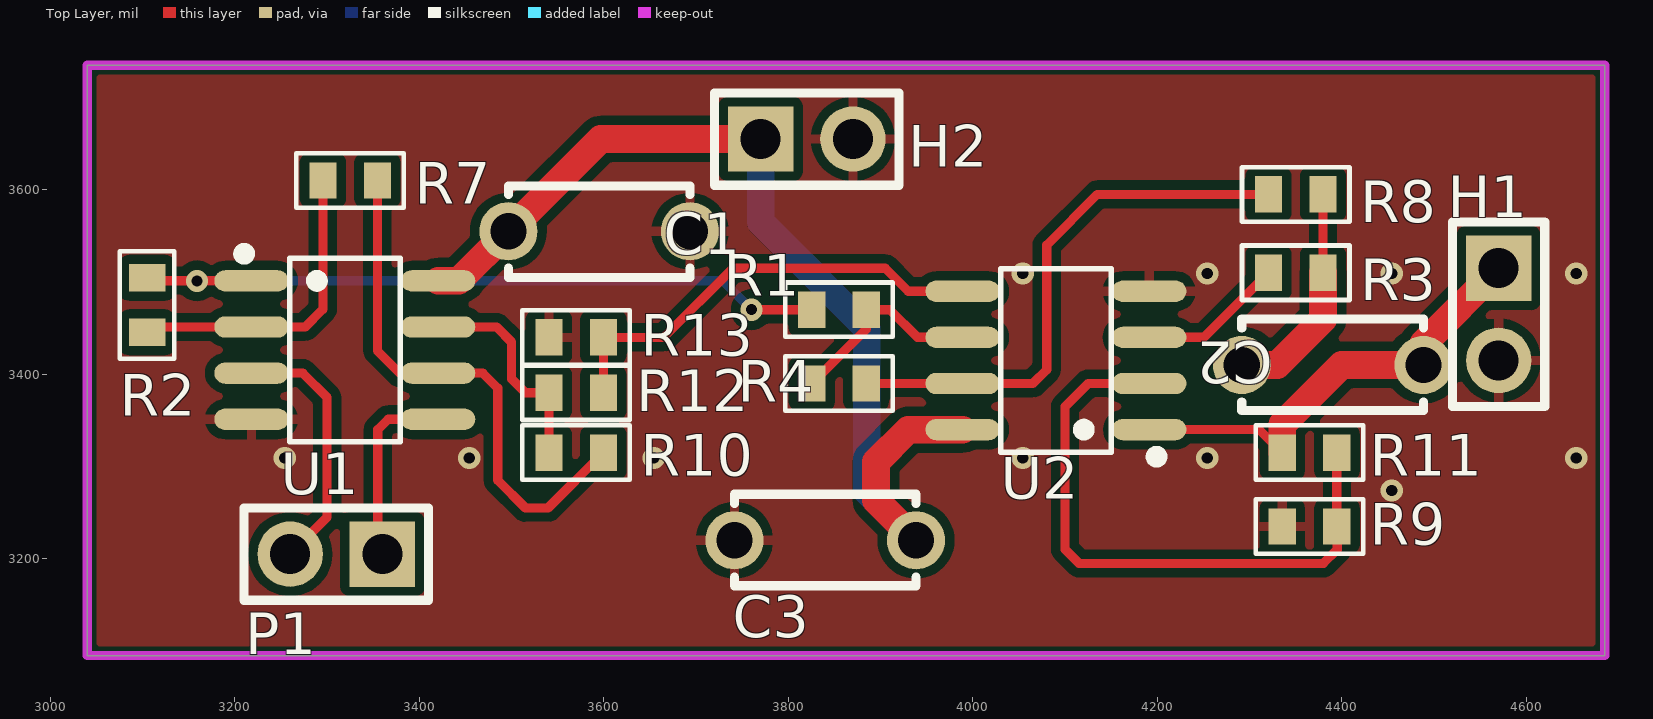
[diagram p0: Top Layer view]
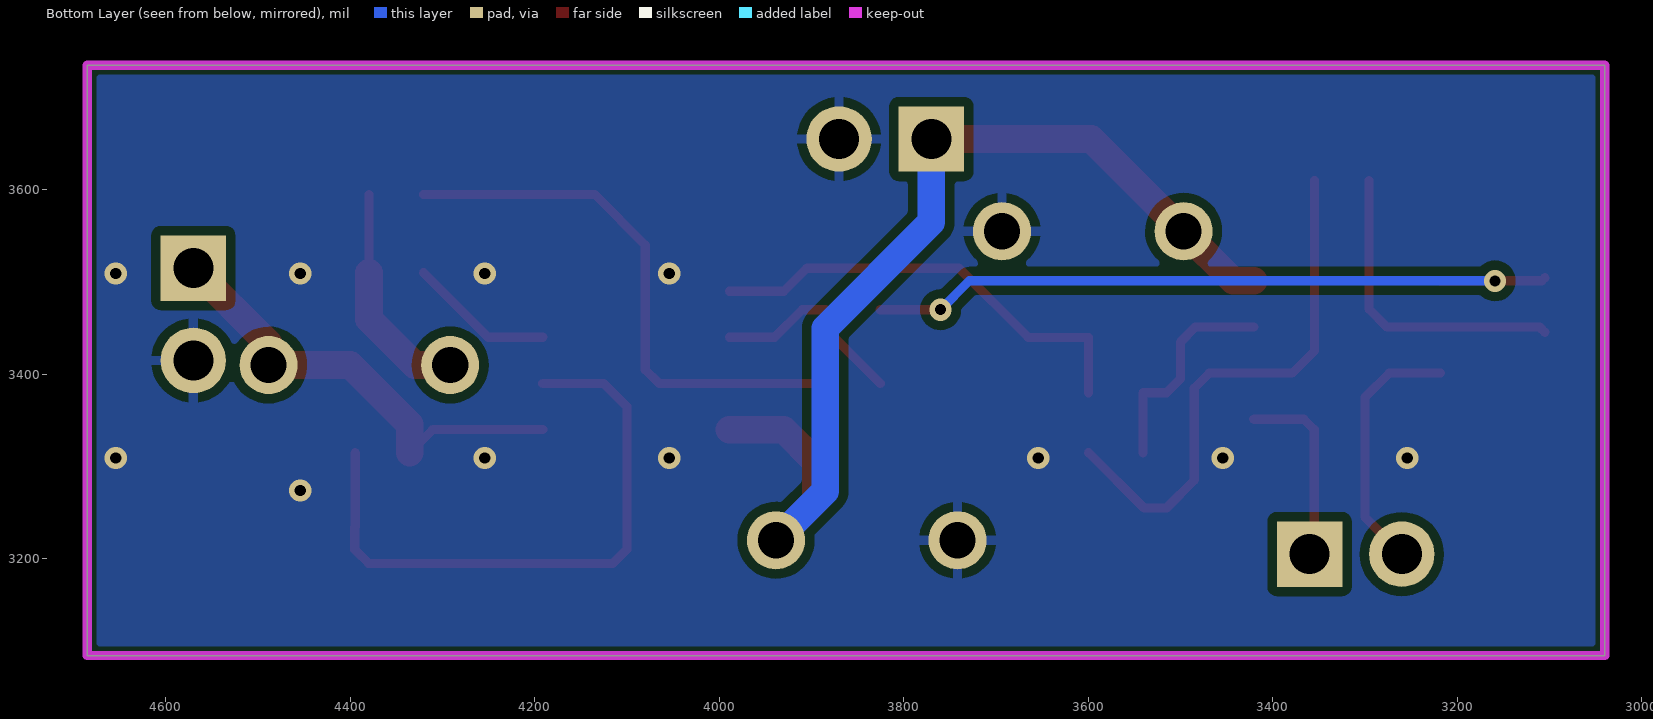
[diagram p1: Bottom Layer view, seen from below]
# Altium PCB MISC49864.pcbdoc
Units mil, origin at the board's own origin, x right, y up, seen from the top; angles counter-clockwise.
Board outline 1645 x 640 mil, 2 copper layers (Top Layer, Bottom Layer), stack 62.206 mil thick; 19 components, 15 nets, 50 pads, 13 vias.

## Layer stack, top to bottom
Top Solder Mask Layer: solder mask 0.394, Dk 3.3
Top Layer: signal copper 1.379
Dielectric1: surface 59.449, FR4, Dk 4.5
Bottom Layer: signal copper 1.378
Bottom Solder Mask Layer: solder mask 0.394, Dk 3.3

## Board outline
3040,3735 3040,3095 4685,3095 4685,3735

## Design rules (kind name [scope] priority, off if disabled: settings)
BoardOutlineClearance copperThickness2oz_1 [All] p2 off: genericclearance=7.99 ignorepadtopadclearanceinfootprint=FALSE except(0: Arc-SplitContinuation Track-SplitContinuation SMDPad-SplitContinuation THPad-SplitContinuation Via-SplitContinuation Fill-SplitContinuation Region-SplitContinuation Poly-SplitContinuation Text-SplitContinuation Hole-SplitContinuation; 5.98: Arc-CutoutEdge SMDPad-CutoutEdge THPad-CutoutEdge Via-CutoutEdge Fill-CutoutEdge Region-CutoutEdge Text-CutoutEdge; 6.93: Hole-OutlineEdge Hole-CutoutEdge; 10: Poly-OutlineEdge Poly-CutoutEdge; 11.81: Arc-OutlineEdge Track-OutlineEdge SMDPad-OutlineEdge THPad-OutlineEdge Via-OutlineEdge Fill-OutlineEdge Region-OutlineEdge Text-OutlineEdge Track-CutoutEdge)
BoardOutlineClearance copperThickness1oz_1 [All] p4: genericclearance=4.02 ignorepadtopadclearanceinfootprint=FALSE except(0: Arc-SplitContinuation Track-SplitContinuation SMDPad-SplitContinuation THPad-SplitContinuation Via-SplitContinuation Fill-SplitContinuation Region-SplitContinuation Poly-SplitContinuation Text-SplitContinuation Hole-SplitContinuation; 6: SMDPad-CutoutEdge THPad-CutoutEdge Via-CutoutEdge Fill-CutoutEdge Region-CutoutEdge Text-CutoutEdge; 6.93: Hole-OutlineEdge Hole-CutoutEdge; 10: Poly-OutlineEdge Poly-CutoutEdge; 11.8: Arc-OutlineEdge Track-OutlineEdge SMDPad-OutlineEdge THPad-OutlineEdge Via-OutlineEdge Fill-OutlineEdge Region-OutlineEdge Text-OutlineEdge; 11.81: Arc-CutoutEdge Track-CutoutEdge)
Clearance copperThickness2oz [All] p1 off: gap=7.99 ignorepadtopadclearanceinfootprint=FALSE except(5.98: SMDPad-Track SMDPad-SMDPad THPad-Track SMDPad-THPad THPad-THPad Track-Via SMDPad-Via THPad-Via Via-Via Fill-Track Region-Track Fill-SMDPad Region-SMDPad Fill-THPad Region-THPad Fill-Via Region-Via Fill-Fill Fill-Region Region-Region Arc-Track Arc-SMDPad Arc-THPad Arc-Via Fill-Arc Region-Arc Arc-Arc Text-Track SMDPad-Text Text-THPad Text-Via Fill-Text Region-Text Arc-Text Text-Text; 6.93: Hole-Track Hole-SMDPad Hole-THPad Hole-Via Fill-Hole Region-Hole Hole-Arc Hole-Text; 10: Poly-Track Poly-SMDPad Poly-THPad Poly-Via Poly-Fill Poly-Region Poly-Poly Poly-Arc Poly-Text Poly-Hole)
Clearance copperThickness1oz [All] p3: gap=4.02 ignorepadtopadclearanceinfootprint=FALSE except(5.98: SMDPad-Track SMDPad-SMDPad THPad-Track SMDPad-THPad THPad-THPad Track-Via SMDPad-Via THPad-Via Via-Via Fill-Track Region-Track Fill-SMDPad Region-SMDPad Fill-THPad Region-THPad Fill-Via Region-Via Fill-Fill Fill-Region Region-Region; 6: Arc-Track Arc-SMDPad Arc-THPad Arc-Via Fill-Arc Region-Arc Arc-Arc Text-Track SMDPad-Text Text-THPad Text-Via Fill-Text Region-Text Arc-Text Text-Text; 6.93: Hole-Track Hole-SMDPad Hole-THPad Hole-Via Fill-Hole Region-Hole Hole-Arc Hole-Text; 10: Poly-Track Poly-SMDPad Poly-THPad Poly-Via Poly-Fill Poly-Region Poly-Poly Poly-Arc Poly-Text Poly-Hole)
DiffPairsRouting differentialPair [All] p1: maxlimit=6 minlimit=6 mostfreqgap=6 toplayer_minwidth=5 toplayer_prefwidth=10 toplayer_maxwidth=100 toplayer_mingap=6 toplayer_prefgap=6 toplayer_maxgap=6 bottomlayer_minwidth=5 bottomlayer_prefwidth=10 bottomlayer_maxwidth=100 bottomlayer_mingap=6 bottomlayer_prefgap=6 bottomlayer_maxgap=6 maxuncoupledlength=10
HoleToHoleClearance otherClearance [All] p1: gap=11.81 allowstackedmicrovias=TRUE
Length netLength [All] p1: minlimit=0 maxlimit=0
MatchedLengths netLengthTolerance [All] p1: tolerance=1000
PasteMaskExpansion pasteMaskExpansion [All] p1: expansion=0
PlaneConnect innerPlane [All] p1: planeconnectstyle=Relief reliefexpansion=20 reliefentries=4 reliefconductorwidth=10 reliefairgap=10
PolygonConnect copperRegion [(InNet('GND'))] p1: connectstyle=Relief reliefconductorwidth=10 reliefentries=4 polygonreliefangle="90 Angle" airgapwidth=10 via.connectstyle=Relief via.reliefconductorwidth=10 via.reliefentries=4 via.polygonreliefangle="90 Angle" via.airgapwidth=10
RoutingVias viaSize [All] p1: holewidth=12.01 width=24.02 viastyle="Through Hole" minholewidth=11.81 minwidth=19.68 maxholewidth=248.03 maxwidth=393.7
SolderMaskExpansion solderMaskExpansion [IsVia] p1: expansion=-1000 istentingtop=TRUE
SolderMaskExpansion solderMaskExpansion [All] p2: expansion=2 istentingtop=FALSE
Width copperThickness2oz_2 [All] p1 off: maxlimit=100 minlimit=8 preferedwidth=10
Width copperThickness1oz_2 [All] p2: maxlimit=100 minlimit=5 preferedwidth=10

## Components (designator, comment, footprint, x,y, rotation, side; value= is the part's Value field where it differs from the comment)
C1 "Cap" CAP-TH_L5.0-W2.5-P5.00-D1.0 3595,3555 r0 top
C2 "Cap" CAP-TH_L5.0-W2.5-P5.00-D1.0 4390,3410 r180 top
C3 "Cap" CAP-TH_L5.0-W2.5-P5.00-D1.0 3840,3220 r180 top
H1 "" HDR-TH_2P-P2.54-V-M-1 4570,3465 r270 top
H2 "" HDR-TH_2P-P2.54-V-M-1 3820,3655 r0 top
P1 "Header 2" HDR-TH_2P-P2.54-V-M-1 3310,3205 r180 top
R1 "10K" R0603_SMD-CRCW060327R0FKEA 3855,3470 r180 top
R2 "10K" R0603_SMD-CRCW060327R0FKEA 3105,3475 r90 top
R3 "1.22K" R0603_SMD-CRCW060327R0FKEA 4350,3510 r180 top
R4 "10K" R0603_SMD-CRCW060327R0FKEA 3855,3390 r180 top
R7 "100" R0603_SMD-CRCW060327R0FKEA 3325,3610 r180 top
R8 "1.22K" R0603_SMD-CRCW060327R0FKEA 4350,3595 r0 top
R9 "4.7K" R0603_SMD-CRCW060327R0FKEA 4365,3235 r0 top
R10 "10K" R0603_SMD-CRCW060327R0FKEA 3570,3315 r0 top
R11 "4.7K" R0603_SMD-CRCW060327R0FKEA 4365,3315 r180 top
R12 "10K" R0603_SMD-CRCW060327R0FKEA 3570,3380 r180 top
R13 "10K" R0603_SMD-CRCW060327R0FKEA 3570,3440 r180 top
U1 "AD8652ARZ" SOIC-8_L4.9-W3.9-P1.27-LS6.0-BL 3319.24,3426.25 r270 top
U2 "AD8652ARZ" SOIC-8_L4.9-W3.9-P1.27-LS6.0-BL 4090,3415 r90 top

## Footprints (in the part's own frame and the unit in brackets; to place one, negate y for a bottom-side part, rotate by r counter-clockwise, add the part's x,y. Pads: shape width x height; smd on the part's side, far side on the other; paste and mask are expansions set on the pad)
CAP-TH_L5.0-W2.5-P5.00-D1.0 [mm]
  round 1.6 hole 1: 1(-2.5,0) 2(2.5,0)
  silkscreen extent -2.5,-1.27 2.5,1.25
HDR-TH_2P-P2.54-V-M-1 [mm]
  rect 1.8x1.8 hole 1.1: 1(-1.27,0)
  round 1.8 hole 1.1: 2(1.27,0)
  silkscreen extent -2.54,-1.27 2.54,1.27
R0603_SMD-CRCW060327R0FKEA [mm]
  rect 0.75x1 smd: 1(-0.75,0) 2(0.75,0)
  silkscreen extent -1.48,-0.75 1.48,0.75
SOIC-8_L4.9-W3.9-P1.27-LS6.0-BL [mm]
  oval 0.588x2.045 smd: 1(-1.905,-2.57) 2(-0.635,-2.57) 3(0.635,-2.57) 4(1.905,-2.57) 5(1.905,2.57) 6(0.635,2.57) 7(-0.635,2.57) 8(-1.905,2.57)
  silkscreen extent -2.8,-2.92 2.53,1.52

## Via types
v1: diameter 24.02, hole 12, Top Layer to Bottom Layer, 13 vias

## Nets (pads, with @x,y where several pads share a name; then routed paths per layer and width w, separated by ;. In a path a pad name is that pad's centre, name@x,y a point inside that pad or via, vN(x,y) a via of type N, cw(c..) or ccw(c..) an arc to the next point about the centre after c; other vN are vias at no path point)
$2N36: R2.1 R7.2 U1.2 | length 340.4
  Top Layer w10: R2.1 3110.78,3451.25 U1.2 3276.25,3451.25 3295.47,3470.47 R7.2
$2N37: R7.1 R10.2 U1.6 | length 583.6
  Top Layer w10: R7.1 3354.53,3425.47 3378.75,3401.25 U1.6 3468.75,3401.25 3485,3385 3485,3285 3515,3255 3539.53,3255 R10.2
$2N38: R1.2 R2.2 U1.1 | length 793.8
  Top Layer w10: R2.2 3108.28,3501.25 v1(3159.03,3501.25) U1.1 ; v1(3760,3470) R1.2
  Bottom Layer w10: v1(3159.03,3501.25) 3728.75,3501.25 v1(3760,3470)
$2N39: R12.1 R13.1 U2.5 | length 490.7
  Top Layer w10: R12.1 R13.1 3665,3440 3740,3515 3905,3515 3930,3490 U2.5
$2N40: R9.2 R11.1 U2.2 | length 669.2
  Top Layer w10: U2.2 4125,3390 4100,3365 4100,3210 4115,3195 4380,3195 4395,3210 4395,3234.53 R9.2 R11.1
$2N41: R3.2 U2.3 | length 158.3
  Top Layer w10: U2.3 4250.47,3440 R3.2
$2N42: R10.1 R12.2 U1.7 | length 238
  Top Layer w10: U1.7 3483.75,3451.25 3500,3435 3500,3395 3515,3380 R12.2 R10.1
$2N43: C2.2 R3.1 R8.2 | length 243.9
  Top Layer w10: R3.1 R8.2
  Top Layer w30: C2.2 4330,3410 4379.53,3459.53 R3.1
$2N46: R1.1 R4.2 U2.6 | length 221.2
  Top Layer w10: R4.2 3884.53,3449.05 R1.1 3910,3470 3940,3440 U2.6
$2N47: R4.1 R8.1 U2.7 | length 599.9
  Top Layer w10: R4.1 U2.7 4065,3390 4080,3405 4080,3540 4135,3595 R8.1
$2N51: P1.1 U1.5 | length 207.2
  Top Layer w10: P1.1 3355,3210 3355,3340 3366.25,3351.25 U1.5
$2N52: P1.2 U1.3 | length 279.4
  Top Layer w10: U1.3 3273.75,3401.25 3300,3375 3300,3245 P1.2
$2N61: C2.1 H1.1 R11.2 U2.1 | length 503.6
  Top Layer w10: U2.1 4310.47,3340 R11.2
  Top Layer w30: R11.2 4335.47,3345.47 4400,3410 C2.1 4488.43,3433.43 H1.1
+5: C1.1 C3.1 H2.1 U1.8 U2.8 | length 1129.3
  Top Layer w30: U1.8 3442.83,3501.25 C1.1 3596.57,3655 H2.1 ; C3.1 3895,3263.43 3895,3305 3930,3340 U2.8
  Bottom Layer w30: H2.1 3770,3565 3885,3450 3885,3273.43 C3.1
GND: C1.2 C3.2 H1.2 H2.2 R9.1 R13.2 U1.4 U2.4
  other v1: 4454.1,3274.1 3254.1,3309.1 3454.1,3309.1 3654.1,3309.1 4054.1,3309.1 4254.1,3309.1 4654.1,3309.1 4054.1,3509.1 4254.1,3509.1 4454.1,3509.1 4654.1,3509.1

## Polygon pours and split planes (outlines as drawn)
GND on Top Layer (solid, remove dead copper, pour order 0): 3000,3815 3000,3000 4705,3000 4705,3815
GND on Bottom Layer (solid, remove dead copper, pour order 2): 3020,3795 3020,3035 4695,3035 4695,3795

## Keep-outs
Board Outline Layer:
  the board outline again, w10